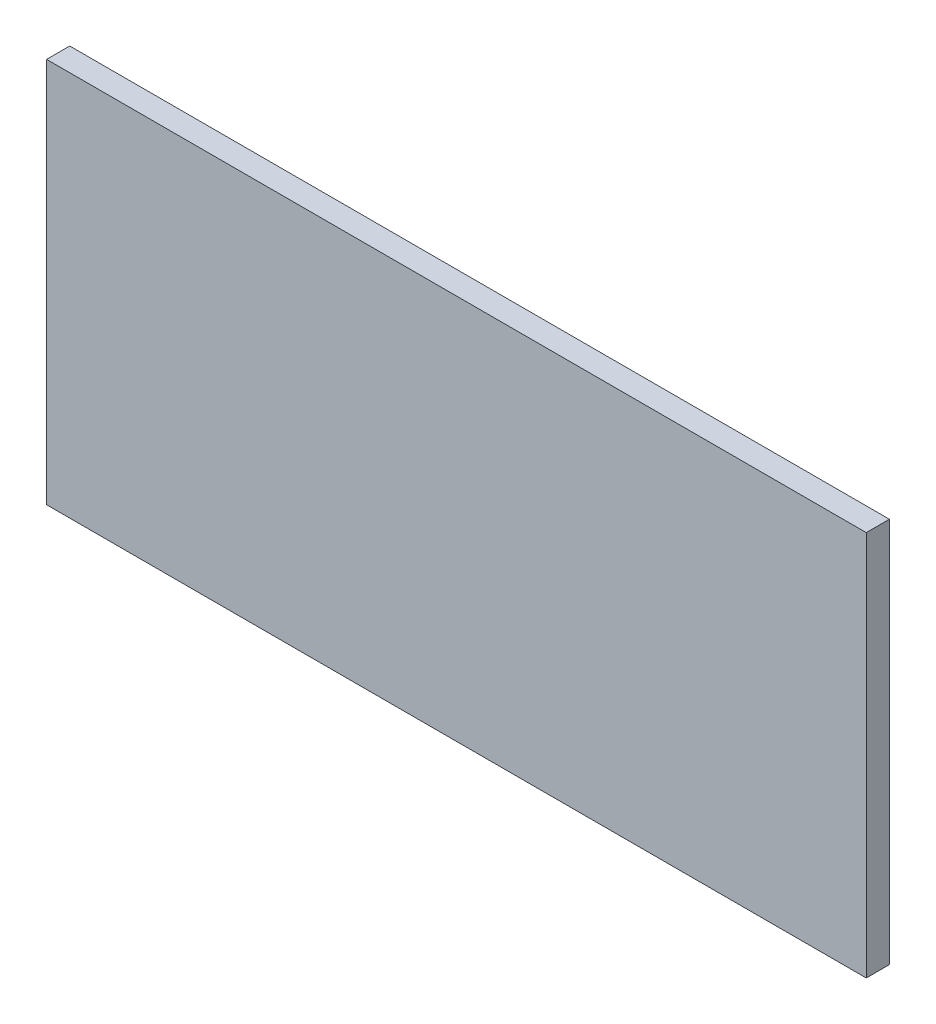
from build123d import *

# Parameters (mm, degrees)
SKETCH1_W           = 425
SKETCH1_H           = 200
BOSS_EXTRUDE1_DEPTH = 12


with BuildPart() as part:
    # Sketch1 → Boss-Extrude1 (new body)
    with BuildSketch(Plane.XY):
        with Locations((212.5, 100)):
            Rectangle(SKETCH1_W, SKETCH1_H)
    extrude(amount=BOSS_EXTRUDE1_DEPTH)


solid = part.part
